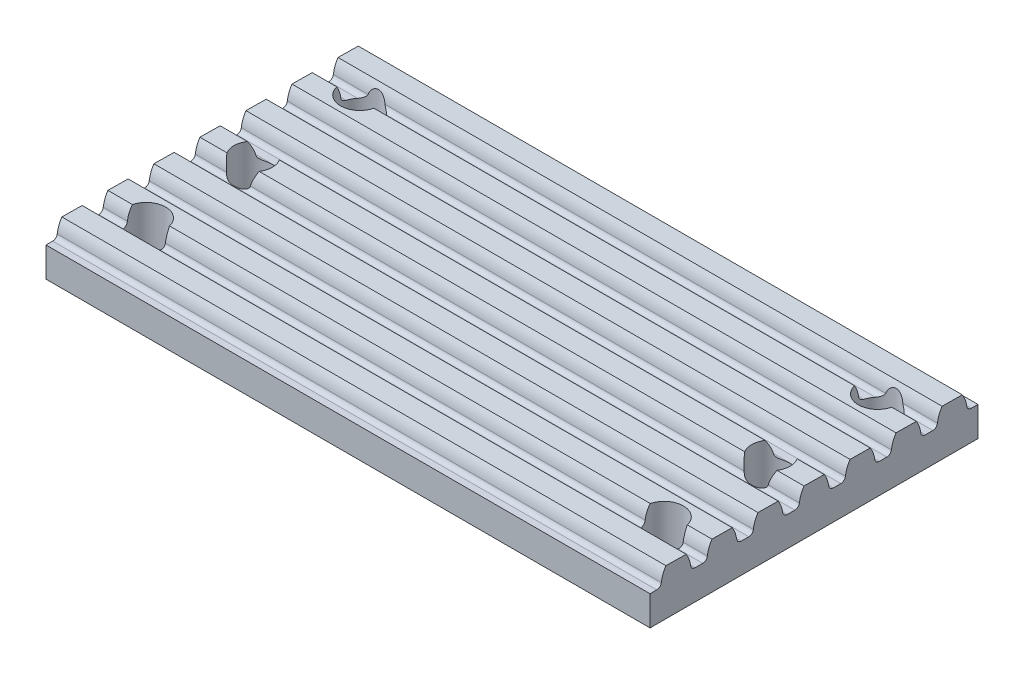
from build123d import *

# Parameters (mm, degrees)
S8M_1_DEPTH        = 105
HOLE_WIZARD_M6_1_D = 6.6


with BuildPart() as part:
    # 草图12 → 其他 S8M压板(1) (new body)
    with BuildSketch(Plane(origin=(0, 0, -28.5), x_dir=(0, 0, -1), z_dir=(1, 0, 0))):
        with BuildLine():
            Line((-27.346312105, 5.15), (-28.5, 5.15))
            Line((-28.5, 5.15), (-28.5, 0))
            Line((-28.5, 0), (28.5, 0))
            Line((28.5, 0), (28.5, 5.15))
            Line((28.5, 5.15), (27.345812084, 5.15))
            ThreePointArc((27.345812084, 5.15), (26.819148277, 5.347816392), (26.552941221, 5.843437072))
            ThreePointArc((26.552941221, 5.843437072), (26.281385905, 6.941041218), (25.778999942, 7.954000001))
            Line((25.778999942, 7.954000001), (22.250668667, 7.999822485))
            ThreePointArc((22.250668667, 7.999822485), (21.727796264, 6.96661325), (21.446541532, 5.843308905))
            ThreePointArc((21.446541532, 5.843308905), (21.18030304, 5.347773774), (20.653687895, 5.15))
            Line((20.653687895, 5.15), (19.345812084, 5.15))
            ThreePointArc((19.345812084, 5.15), (18.819148277, 5.347816392), (18.552941221, 5.843437072))
            ThreePointArc((18.552941221, 5.843437072), (18.281385905, 6.941041218), (17.778999942, 7.954000001))
            Line((17.778999942, 7.954000001), (14.250668667, 7.999822485))
            ThreePointArc((14.250668667, 7.999822485), (13.727796264, 6.96661325), (13.446541532, 5.843308905))
            ThreePointArc((13.446541532, 5.843308905), (13.18030304, 5.347773774), (12.653687895, 5.15))
            Line((12.653687895, 5.15), (11.345812084, 5.15))
            ThreePointArc((11.345812084, 5.15), (10.819148277, 5.347816392), (10.552941221, 5.843437072))
            ThreePointArc((10.552941221, 5.843437072), (10.281385905, 6.941041218), (9.778999942, 7.954000001))
            Line((9.778999942, 7.954000001), (6.250668667, 7.999822485))
            ThreePointArc((6.250668667, 7.999822485), (5.727796264, 6.96661325), (5.446541532, 5.843308905))
            ThreePointArc((5.446541532, 5.843308905), (5.18030304, 5.347773774), (4.653687895, 5.15))
            Line((4.653687895, 5.15), (3.345812084, 5.15))
            ThreePointArc((3.345812084, 5.15), (2.819148277, 5.347816392), (2.552941221, 5.843437072))
            ThreePointArc((2.552941221, 5.843437072), (2.281385905, 6.941041218), (1.778999942, 7.954000001))
            Line((1.778999942, 7.954000001), (-1.749331333, 7.999822485))
            ThreePointArc((-1.749331333, 7.999822485), (-2.272203736, 6.96661325), (-2.553458468, 5.843308905))
            ThreePointArc((-2.553458468, 5.843308905), (-2.81969696, 5.347773774), (-3.346312105, 5.15))
            Line((-3.346312105, 5.15), (-4.654187916, 5.15))
            ThreePointArc((-4.654187916, 5.15), (-5.180851723, 5.347816392), (-5.447058779, 5.843437072))
            ThreePointArc((-5.447058779, 5.843437072), (-5.718614095, 6.941041218), (-6.221000058, 7.954000001))
            Line((-6.221000058, 7.954000001), (-9.749331333, 7.999822485))
            ThreePointArc((-9.749331333, 7.999822485), (-10.272203736, 6.96661325), (-10.553458468, 5.843308905))
            ThreePointArc((-10.553458468, 5.843308905), (-10.81969696, 5.347773774), (-11.346312105, 5.15))
            Line((-11.346312105, 5.15), (-12.654187916, 5.15))
            ThreePointArc((-12.654187916, 5.15), (-13.180851723, 5.347816392), (-13.447058779, 5.843437072))
            ThreePointArc((-13.447058779, 5.843437072), (-13.718614095, 6.941041218), (-14.221000058, 7.954000001))
            Line((-14.221000058, 7.954000001), (-17.749331333, 7.999822485))
            ThreePointArc((-17.749331333, 7.999822485), (-18.272203736, 6.96661325), (-18.553458468, 5.843308905))
            ThreePointArc((-18.553458468, 5.843308905), (-18.81969696, 5.347773774), (-19.346312105, 5.15))
            Line((-19.346312105, 5.15), (-20.654187916, 5.15))
            ThreePointArc((-20.654187916, 5.15), (-21.180851723, 5.347816392), (-21.447058779, 5.843437072))
            ThreePointArc((-21.447058779, 5.843437072), (-21.718614095, 6.941041218), (-22.221000058, 7.954000001))
            Line((-22.221000058, 7.954000001), (-25.749331333, 7.999822485))
            ThreePointArc((-25.749331333, 7.999822485), (-26.272203736, 6.96661325), (-26.553458468, 5.843308905))
            ThreePointArc((-26.553458468, 5.843308905), (-26.81969696, 5.347773774), (-27.346312105, 5.15))
        make_face()
    extrude(amount=S8M_1_DEPTH)

    # M6 间隙孔1 (through all)
    with Locations(Plane(origin=(0, 0, 0), x_dir=(-1, 0, 0), z_dir=(0, -1, 0))):
        with Locations((-7.5, 10), (-7.5, 47), (-97.5, 47), (-97.5, 10), (-97.5, 28.5), (-7.5, 28.5)):
            Hole(HOLE_WIZARD_M6_1_D / 2)


solid = part.part
